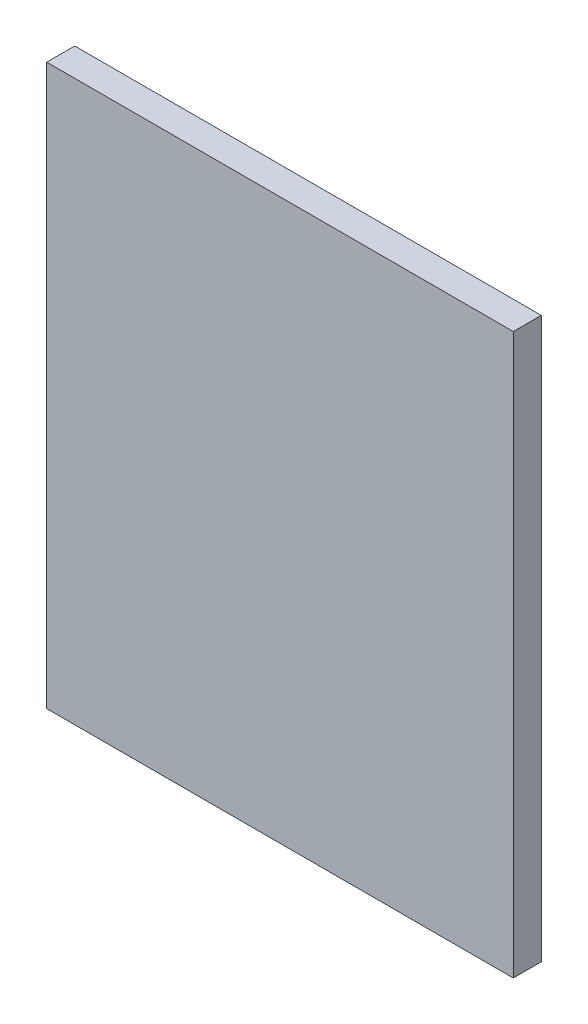
SolidWorks part; units mm, degrees
ref_plane "前视基准面" through (0, 0, 0) normal (0, 0, 1) x (1, 0, 0)
ref_plane "上视基准面" through (0, 0, 0) normal (0, 1, 0) x (1, 0, 0)
ref_plane "右视基准面" through (0, 0, 0) normal (1, 0, 0) x (0, 0, -1)
sketch "草图1" plane through (0, 0, 0) normal (0, 0, 1) x (1, 0, 0)
  line L0 (0, 0) -> (0, 120)
  line L1 (0, 120) -> (100, 120)
  line L2 (100, 120) -> (100, 0)
  line L3 (100, 0) -> (0, 0)
extrude "凸台-拉伸1" add sketch "草图1" along normal blind 6
